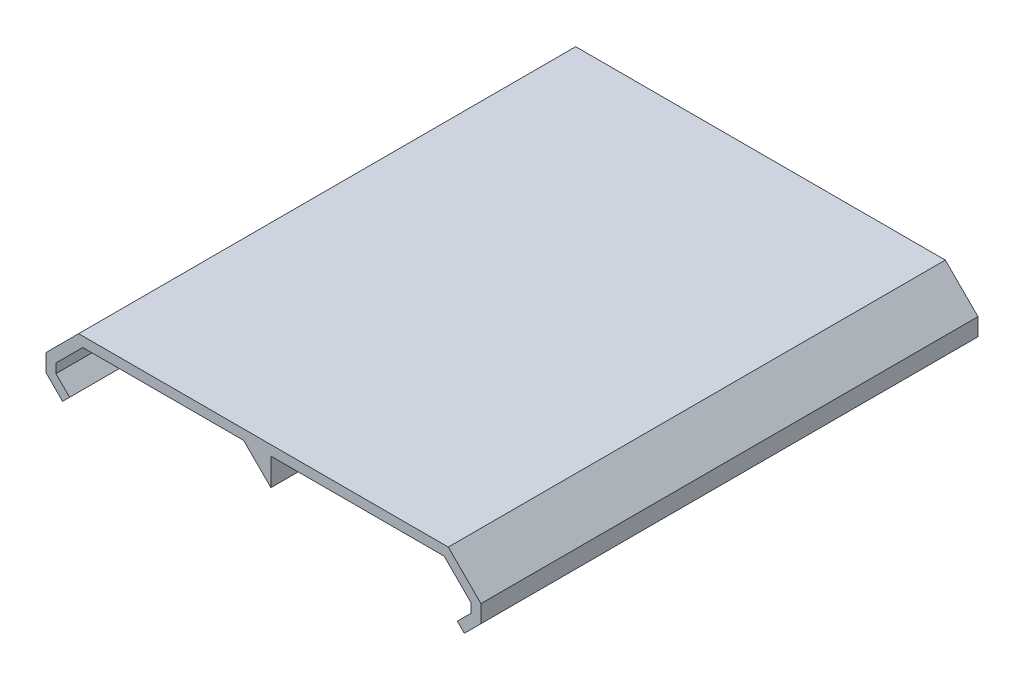
SolidWorks part; units mm, degrees
ref_plane "Front Plane" through (0, 0, 0) normal (0, 0, 1) x (1, 0, 0)
ref_plane "Top Plane" through (0, 0, 0) normal (0, 1, 0) x (1, 0, 0)
ref_plane "Right Plane" through (0, 0, 0) normal (1, 0, 0) x (0, 0, -1)
sketch "Sketch1" plane through (0, 0, 0) normal (0, 0, 1) x (1, 0, 0)
  line L0 (0, 0) -> (0, 52) construction
  line L1 (72.7071, 52) -> (-72.7071, 52)
  line L2 (-72.7071, 52) -> (-83.5, 41.2071)
  line L3 (-83.5, 41.2071) -> (-83.5, 37.5)
  line L4 (-83.5, 37.5) -> (-78, 32)
  line L10 (83.5, 37.5) -> (78, 32)
  line L11 (83.5, 41.2071) -> (83.5, 37.5)
  line L12 (72.7071, 52) -> (83.5, 41.2071)
extrude "Extrude-Thin1" add sketch "Sketch1" against normal blind 200 thin
sketch "Sketch2" plane through (0, 0, 0) normal (0, 0, 1) x (1, 0, 0)
  line L0 (-7.9899, 52) -> (3, 52)
  line L1 (-72.7071, 52) -> (72.7071, 52) construction
  line L2 (3, 52) -> (3, 41.0101)
  line L3 (3, 41.0101) -> (-7.9899, 52)
  line L5 (3, 20.8) -> (3, 0) construction
  line L6 (-4.4042, 47) -> (3, 39.5958) construction
  dimension "D1" = 1
extrude "Boss-Extrude1" add sketch "Sketch2" against normal blind 37
